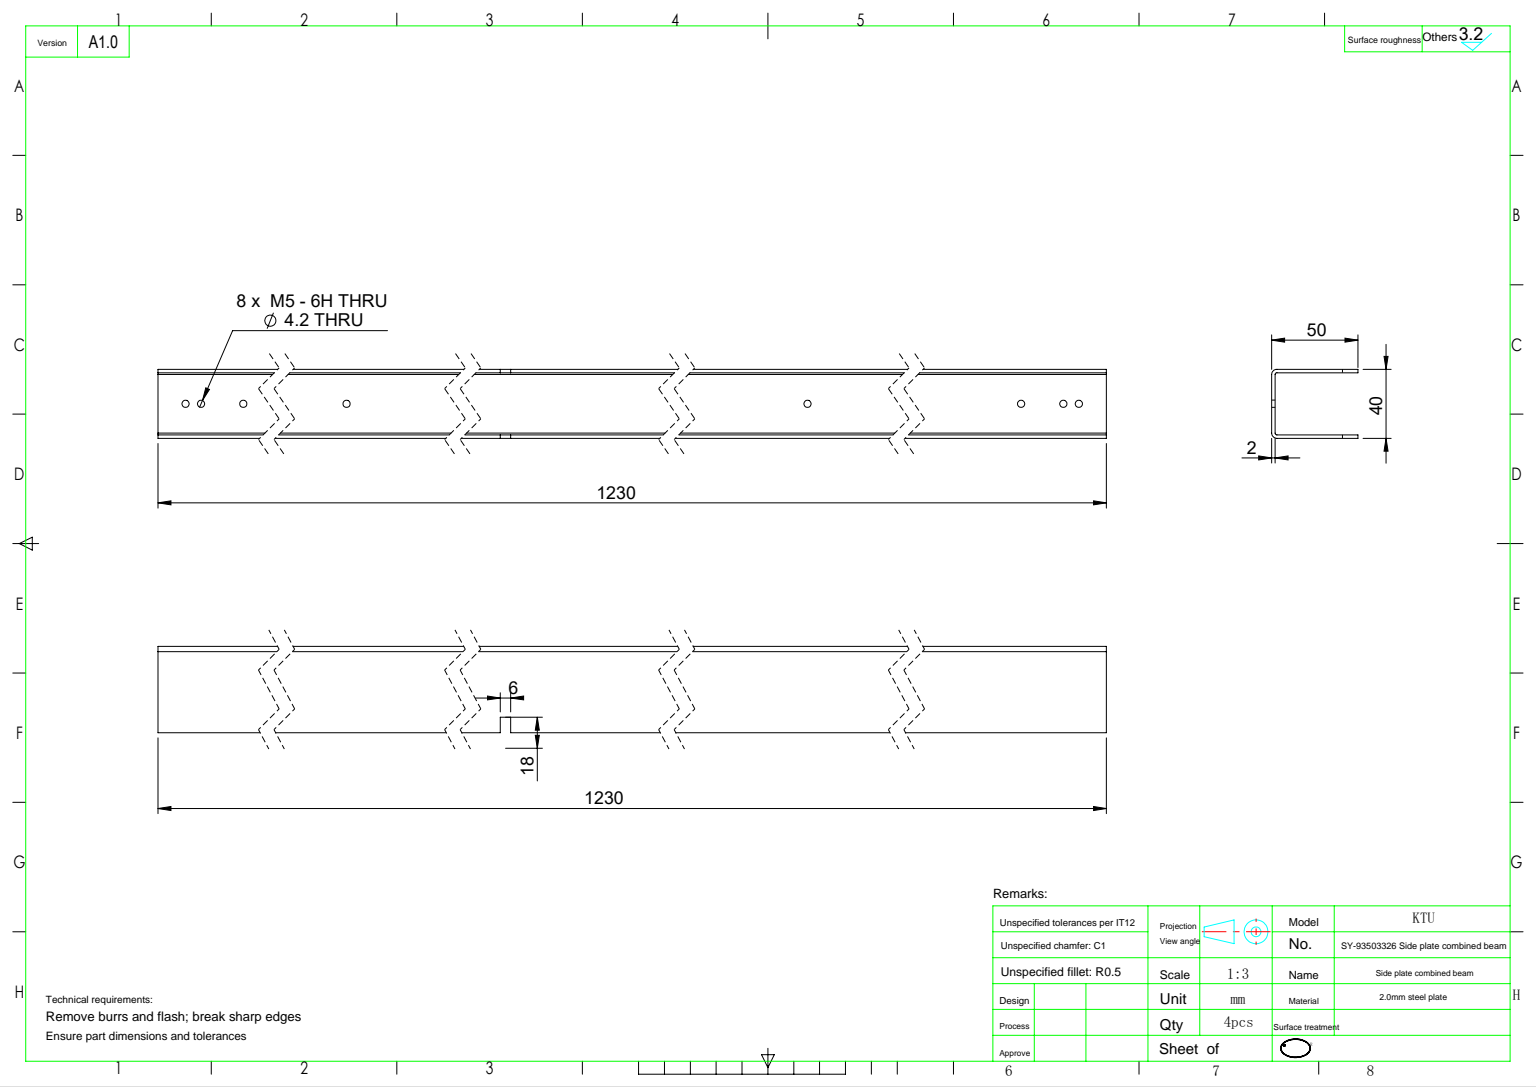
SolidWorks part; units mm, degrees
ref_plane "前视基准面" through (0, 0, 0) normal (0, 0, 1) x (1, 0, 0)
ref_plane "上视基准面" through (0, 0, 0) normal (0, 1, 0) x (1, 0, 0)
ref_plane "右视基准面" through (0, 0, 0) normal (1, 0, 0) x (0, 0, -1)
sketch "草图1" plane through (0, 0, 0) normal (0, 0, 1) x (1, 0, 0)
  line L1 (-22, 20) -> (25, 20)
  line L2 (-25, 17) -> (-25, -17)
  line L3 (-22, -20) -> (25, -20)
  line L5 (-25, 20) -> (25, -20) construction
  line L6 (-25, -20) -> (25, 20) construction
  arc A2 (-25, -17) -> (-22, -20) centre (-22, -17) ccw
  arc A3 (-22, 20) -> (-25, 17) centre (-22, 17) ccw
  point P0 (0, 0)
  dimension "D3" = 50
  dimension "D4" = 3
  dimension "D1" = 50
  dimension "D2" = 40
extrude "拉伸-薄壁1" add sketch "草图1" along normal mid plane 1230 thin
sketch "草图2" plane through (0, -20, 0) normal (0, -1, 0) x (1, 0, 0)
  line L0 (0, 0) -> (25, 0) construction
  line L2 (25, 615) -> (25, -615) construction
  line L3 (34, 42) -> (16, 42)
  line L4 (34, 42) -> (34, 48)
  line L5 (34, 48) -> (16, 48)
  line L6 (16, 42) -> (16, 48)
  line L7 (34, 42) -> (16, 48) construction
  line L8 (34, 48) -> (16, 42) construction
  point P10 (25, 45)
  dimension "D1" = 6
  dimension "D2" = 18
  dimension "D3" = 9
  dimension "D4" = 45
extrude "切除-拉伸1" cut sketch "草图2" against normal through all
hole_wizard "M5 螺纹孔1" positions "草图3" profile "草图4" tap size "M5" standard "GB" end condition up to next
sketch "草图3" plane through (-25, 0, 0) normal (-1, 0, 0) x (0, 0, 1)
  line L0 (615, 17) -> (615, -17) construction
  line L1 (0, 0) -> (0, 116.9173) construction
  line L2 (599, 0) -> (615, 0) construction
  line L4 (565.5, 0) -> (599, 0) construction
  point P3 (590, 0)
  point P5 (320, 0)
  point P15 (-320, 0)
  point P16 (-590, 0)
  point P17 (565.5, 0)
  point P19 (599, 0)
  point P23 (-599, 0)
  point P24 (-565.5, 0)
  dimension "D1" = 25
  dimension "D2" = 270
  dimension "D3" = 16
  dimension "D4" = 33.5
sketch "草图4" plane through (-25, 0, 590) normal (0, 1, 0) x (0, 0, 1)
  line L0 (0, 0) -> (0, 2)
  line L1 (0, 2) -> (2.1, 2)
  line L2 (2.1, 2) -> (2.1, 0)
  line L5 (2.1, 0) -> (0, 0)
  line L11 (0, -6.35) -> (0, 107.95) construction
  dimension "螺纹线主直径" = 4.2
  dimension "通孔螺纹孔钻头深度" = 2
